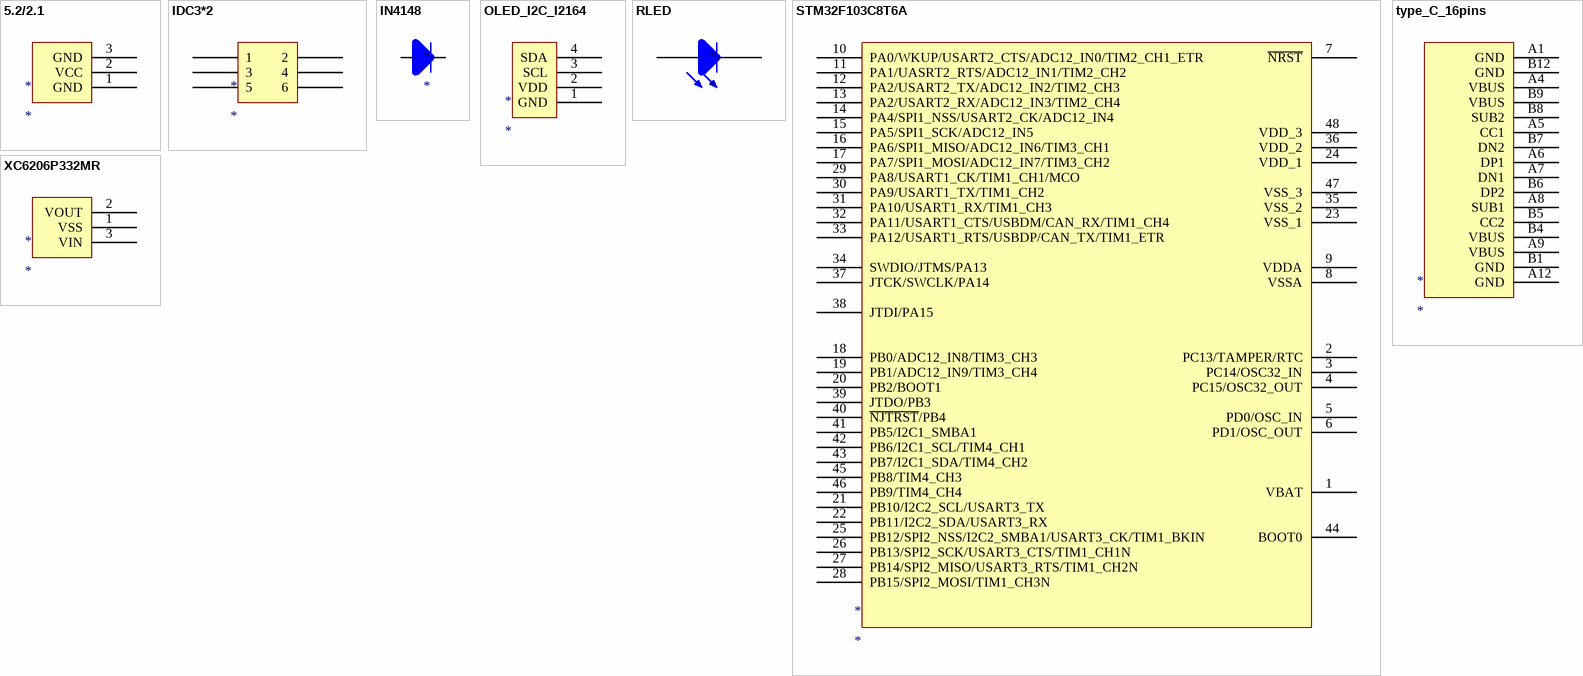
[diagram p0: symbols 5.2/2.1 to XC6206P332MR]
# Altium schematic symbol library MISC82121-9.SchLib: 8 symbols
Pins are listed as number, name and electrical type; pins without a type are passive.


## 5.2/2.1
designator *
pins: 1 GND, 2 VCC, 3 GND

## IDC3*2
designator *
pins: 1, 2, 3, 4, 5, 6

## IN4148
designator *
pins: B14, B15

## OLED_I2C_I2164
designator *
pins: 1 GND, 2 VDD, 3 SCL, 4 SDA

## RLED
designator *
pins: B14, B15

## STM32F103C8T6A
designator *
pins: 1 VBAT, 2 PC13/TAMPER/RTC, 3 PC14/OSC32_IN, 4 PC15/OSC32_OUT, 5 PD0/OSC_IN, 6 PD1/OSC_OUT, 7 ~{NRST}, 8 VSSA, 9 VDDA, 10 PA0/WKUP/USART2_CTS/ADC12_IN0/TIM2_CH1_ETR, 11 PA1/UASRT2_RTS/ADC12_IN1/TIM2_CH2, 12 PA2/USART2_TX/ADC12_IN2/TIM2_CH3, 13 PA2/USART2_RX/ADC12_IN3/TIM2_CH4, 14 PA4/SPI1_NSS/USART2_CK/ADC12_IN4, 15 PA5/SPI1_SCK/ADC12_IN5, 16 PA6/SPI1_MISO/ADC12_IN6/TIM3_CH1, 17 PA7/SPI1_MOSI/ADC12_IN7/TIM3_CH2, 18 PB0/ADC12_IN8/TIM3_CH3, 19 PB1/ADC12_IN9/TIM3_CH4, 20 PB2/BOOT1, 21 PB10/I2C2_SCL/USART3_TX, 22 PB11/I2C2_SDA/USART3_RX, 23 VSS_1, 24 VDD_1, 25 PB12/SPI2_NSS/I2C2_SMBA1/USART3_CK/TIM1_BKIN, 26 PB13/SPI2_SCK/USART3_CTS/TIM1_CH1N, 27 PB14/SPI2_MISO/USART3_RTS/TIM1_CH2N, 28 PB15/SPI2_MOSI/TIM1_CH3N, 29 PA8/USART1_CK/TIM1_CH1/MCO, 30 PA9/USART1_TX/TIM1_CH2, 31 PA10/USART1_RX/TIM1_CH3, 32 PA11/USART1_CTS/USBDM/CAN_RX/TIM1_CH4, 33 PA12/USART1_RTS/USBDP/CAN_TX/TIM1_ETR, 34 SWDIO/JTMS/PA13, 35 VSS_2, 36 VDD_2, 37 JTCK/SWCLK/PA14, 38 JTDI/PA15, 39 JTDO/PB3, 40 ~{NJTRST}/PB4, 41 PB5/I2C1_SMBA1, 42 PB6/I2C1_SCL/TIM4_CH1, 43 PB7/I2C1_SDA/TIM4_CH2, 44 BOOT0, 45 PB8/TIM4_CH3, 46 PB9/TIM4_CH4, 47 VSS_3, 48 VDD_3

## type_C_16pins
designator *
pins: A1 GND, A4 VBUS, A5 CC1, A6 DP1, A7 DN1, A8 SUB1, A9 VBUS, A12 GND, B1 GND, B4 VBUS, B5 CC2, B6 DP2, B7 DN2, B8 SUB2, B9 VBUS, B12 GND

## XC6206P332MR
designator *
pins: 1 VSS, 2 VOUT, 3 VIN